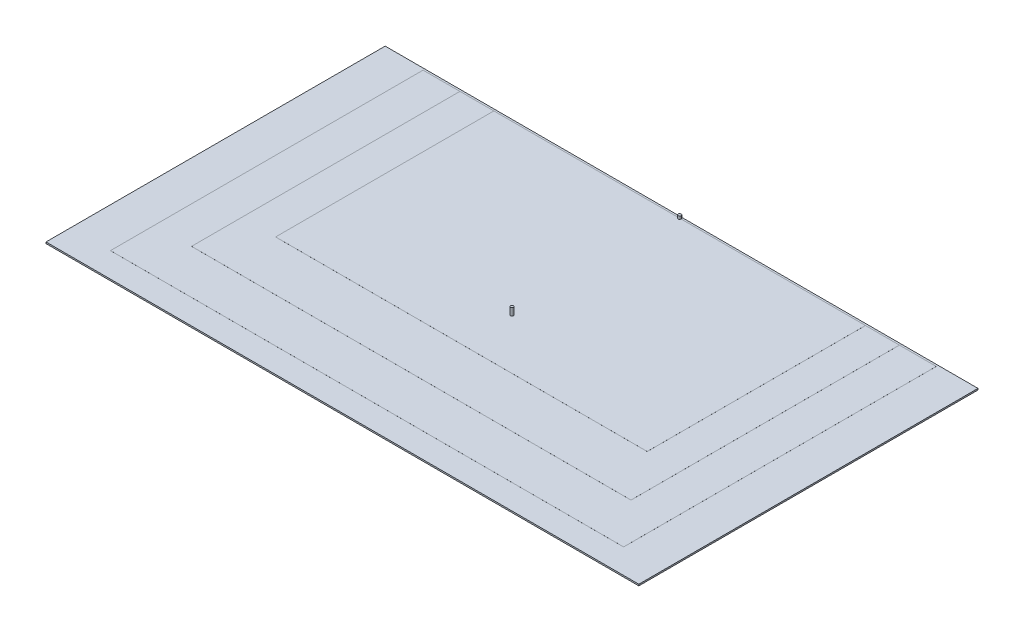
SolidWorks part; units mm, degrees
material "亚克力"
ref_plane "前基準面" through (0, 0, 0) normal (0, 0, 1) x (1, 0, 0)
ref_plane "上基準面" through (0, 0, 0) normal (0, 1, 0) x (1, 0, 0)
ref_plane "右基準面" through (0, 0, 0) normal (1, 0, 0) x (0, 0, -1)
sketch "草图1" plane through (0, 0, 0) normal (0, 1, 0) x (1, 0, 0)
  line L1 (-1005, -575) -> (1005, -575)
  line L2 (-1005, -575) -> (-1005, 575)
  line L3 (-1005, 575) -> (1005, 575)
  line L4 (1005, -575) -> (1005, 575)
  line L5 (-1005, -575) -> (1005, 575) construction
  line L6 (-1005, 575) -> (1005, -575) construction
  point P0 (0, 0)
  dimension "D1" = 2010
  dimension "D2" = 1150
extrude "凸台-拉伸1" add sketch "草图1" along normal mid plane 5
sketch "草图2" plane through (0, 2.5, 0) normal (0, 1, 0) x (1, 0, 0)
  line L0 (1005, 575) -> (-1005, 575) construction
  line L1 (-997.5, -675) -> (997.5, -675)
  line L2 (-997.5, -675) -> (-997.5, 575)
  line L3 (-997.5, 575) -> (997.5, 575)
  line L4 (997.5, -675) -> (997.5, 575)
  line L5 (-997.5, -675) -> (997.5, 575) construction
  line L6 (-997.5, 575) -> (997.5, -675) construction
  point P0 (0, -50)
  dimension "D1" = 1995
  dimension "D2" = 1250
sketch "草图3" plane through (0, 2.6, 0) normal (0, 1, 0) x (1, 0, 0)
  line L0 (997.5, 568.5) -> (-997.5, 568.5) construction
  line L1 (-870, -491.5) -> (870, -491.5)
  line L2 (-870, -491.5) -> (-870, 568.5)
  line L3 (-870, 568.5) -> (870, 568.5)
  line L4 (870, -491.5) -> (870, 568.5)
  line L5 (-870, -491.5) -> (870, 568.5) construction
  line L6 (-870, 568.5) -> (870, -491.5) construction
  point P0 (0, 38.5)
  dimension "D1" = 1740
  dimension "D2" = 1060
extrude "凸台-拉伸5" add sketch "草图3" along normal blind 0.1 separate body
sketch "草图4" plane through (0, 2.7, 0) normal (0, 1, 0) x (1, 0, 0)
  line L0 (870, 568.5) -> (-870, 568.5) construction
  line L1 (-745, -341.5) -> (745, -341.5)
  line L2 (-745, -341.5) -> (-745, 568.5)
  line L3 (-745, 568.5) -> (745, 568.5)
  line L4 (745, -341.5) -> (745, 568.5)
  line L5 (-745, -341.5) -> (745, 568.5) construction
  line L6 (-745, 568.5) -> (745, -341.5) construction
  point P0 (0, 113.5)
  dimension "D1" = 1490
  dimension "D2" = 910
extrude "凸台-拉伸6" add sketch "草图4" along normal blind 0.1 separate body
sketch "草图5" plane through (0, 2.8, 0) normal (0, 1, 0) x (1, 0, 0)
  line L0 (745, 568.5) -> (-745, 568.5) construction
  line L1 (-630, -171.5) -> (630, -171.5)
  line L2 (-630, -171.5) -> (-630, 568.5)
  line L3 (-630, 568.5) -> (630, 568.5)
  line L4 (630, -171.5) -> (630, 568.5)
  line L5 (-630, -171.5) -> (630, 568.5) construction
  line L6 (-630, 568.5) -> (630, -171.5) construction
  point P0 (0, 198.5)
  dimension "D1" = 1260
  dimension "D2" = 740
extrude "凸台-拉伸7" add sketch "草图5" along normal blind 0.1 separate body
sketch "草图6" plane through (0, 2.9, 0) normal (0, 1, 0) x (1, 0, 0)
  circle A0 centre (0, 0) radius 5
  dimension "D1" = 10
extrude "凸台-拉伸8" add sketch "草图6" along normal mid plane 50
sketch "草图7" plane through (0, 2.9, 0) normal (0, 1, 0) x (1, 0, 0)
  line L0 (630, 568.5) -> (-630, 568.5) construction
  circle A0 centre (0, 568.5) radius 5
  dimension "D1" = 10
extrude "凸台-拉伸9" add sketch "草图7" along normal blind 10
